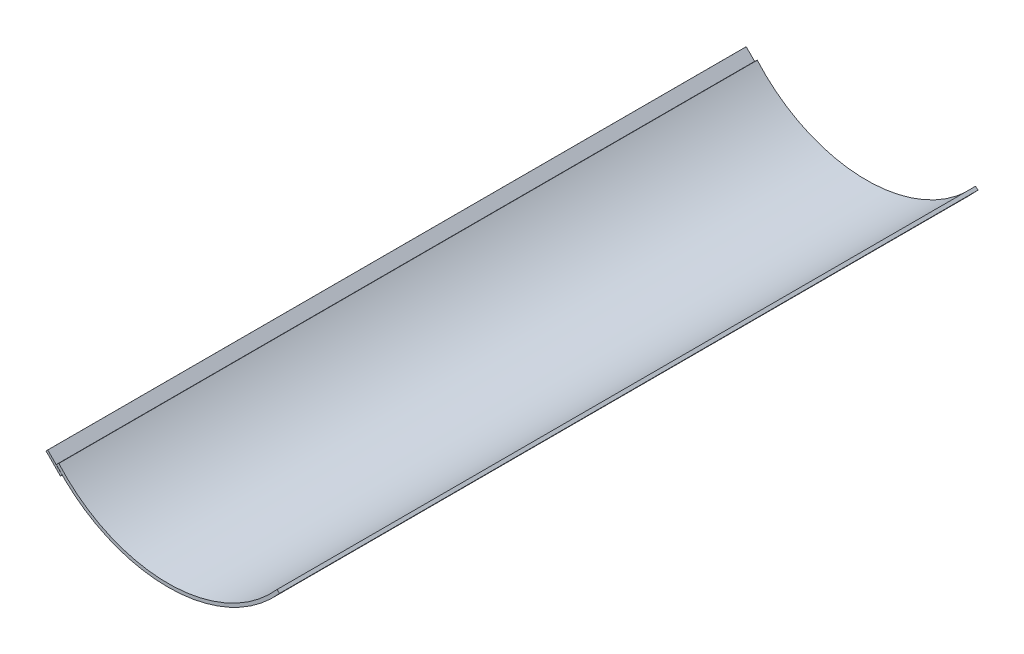
from build123d import *

# Parameters (mm, degrees)
EXTRUDE_1_DEPTH   = 425
EXTRUDE_1_2_DEPTH = 850


with BuildPart() as part:
    # 草图1 → Extrude 1 (new, symmetric)
    with BuildSketch(Plane.XY):
        with BuildLine():
            ThreePointArc((-132.815661727, -117), (0, -177), (132.815661727, -117))
            Line((132.815661727, -117), (135.817145608, -119.644067797))
            ThreePointArc((135.817145608, -119.644067797), (0, -181), (-135.817145608, -119.644067797))
            Line((-135.817145608, -119.644067797), (-132.815661727, -117))
        make_face()
    extrude(amount=EXTRUDE_1_DEPTH, both=True)


with BuildPart() as body_2:
    # 草图2 → Extrude 1 2 (new, through all)
    with BuildSketch(Plane(origin=(0, 0, -425), x_dir=(-1, 0, 0), z_dir=(0, 0, -1))):
        Polygon((146.258901195, -109.518645999), (128.677169739, -127.291735742), (130.809940508, -129.401543516), (148.391671964, -111.628453773), align=None)
    extrude(amount=-EXTRUDE_1_2_DEPTH)


solid = Compound([part.part, body_2.part])
